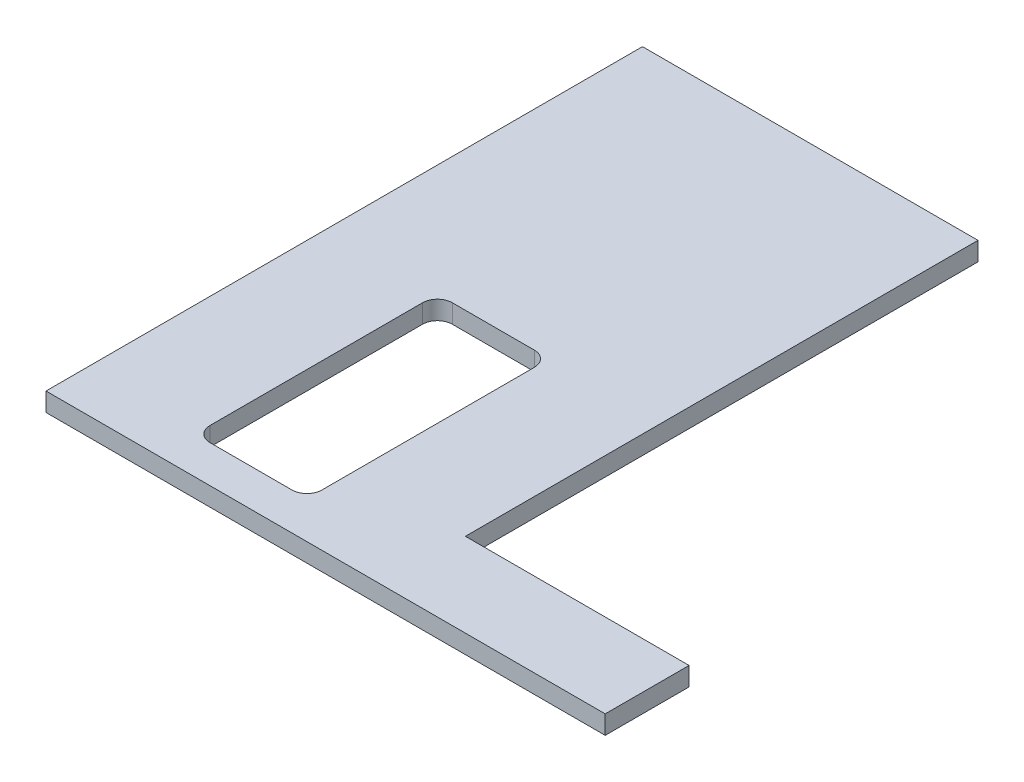
from build123d import *

# Parameters (mm, degrees)
SKETCH1_W           = 180
SKETCH1_H           = 320
BOSS_EXTRUDE1_DEPTH = 10
SKETCH2_W           = 60
SKETCH2_H           = 130
CUT_EXTRUDE1_DEPTH  = 184.847763109
FILLET1_R           = 8
SKETCH3_W           = 45
SKETCH3_H           = 10
BOSS_EXTRUDE2_DEPTH = 120


with BuildPart() as part:
    # Sketch1 → Boss-Extrude1 (new body)
    with BuildSketch(Plane(origin=(0, 0, 0), x_dir=(1, 0, 0), z_dir=(0, 1, 0))):
        Rectangle(SKETCH1_W, SKETCH1_H)
    extrude(amount=BOSS_EXTRUDE1_DEPTH)

    # Sketch2 → Cut-Extrude1 (cut, through all)
    with BuildSketch(Plane(origin=(0, 10, 0), x_dir=(1, 0, 0), z_dir=(0, 1, 0))):
        with Locations((0, -75)):
            Rectangle(SKETCH2_W, SKETCH2_H)
    extrude(amount=-CUT_EXTRUDE1_DEPTH, mode=Mode.SUBTRACT)

    # Fillet1
    fillet1_edges = [part.edges().sort_by_distance(p)[0] for p in [
        (30, 5, 10),
        (30, 5, 140),
        (-30, 5, 140),
        (-30, 5, 10),
    ]]
    fillet(fillet1_edges, radius=FILLET1_R)

    # Sketch3 → Boss-Extrude2 (add)
    with BuildSketch(Plane(origin=(90, 0, 0), x_dir=(0, 0, -1), z_dir=(1, 0, 0))):
        with Locations((-137.5, 5)):
            Rectangle(SKETCH3_W, SKETCH3_H)
    extrude(amount=BOSS_EXTRUDE2_DEPTH)


solid = part.part
